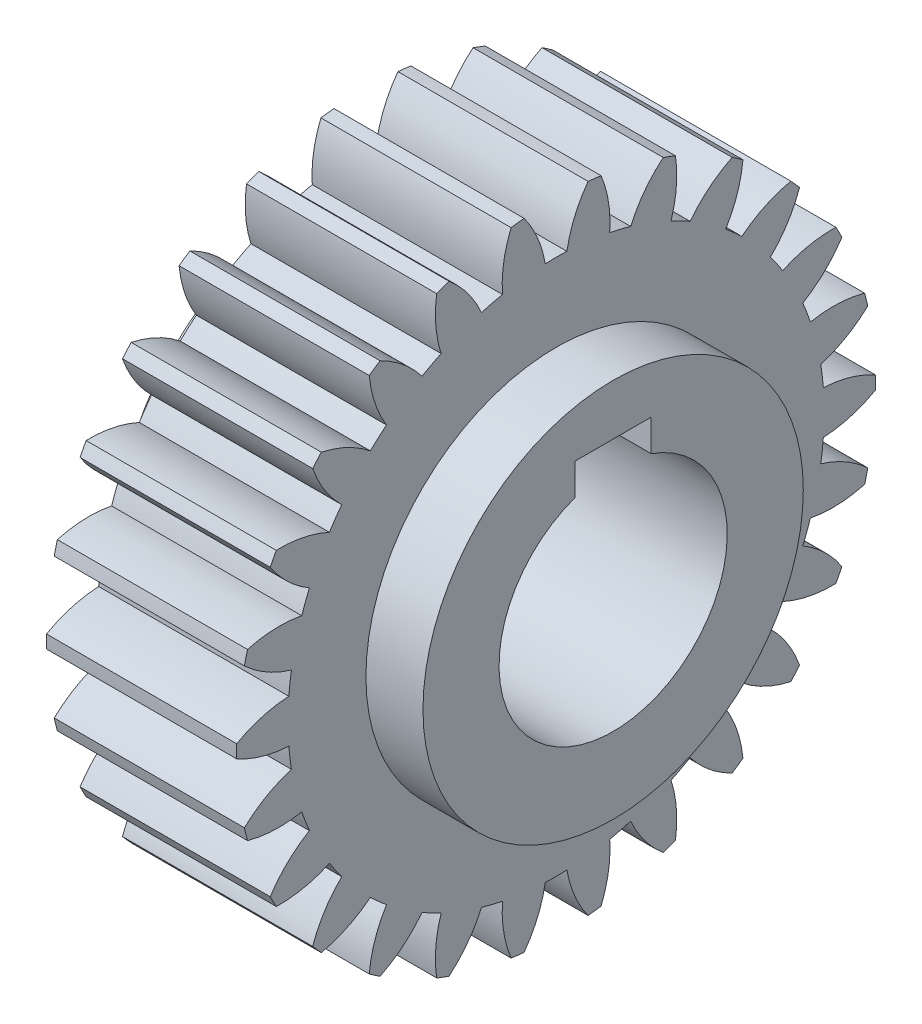
from build123d import *

# Parameters (mm, degrees)
BASPROSKE_W       = 25
BASPROSKE_H       = 42
TOOTHCUT_DEPTH    = 65.443773943
TEETHCUTS_COUNT   = 26
TEETHCUTS_ANGLE   = 346.153846154
HUBNEABOTSKE_R    = 25
HUBNEARBOTH_DEPTH = 7.5000254
HUBFAR_START      = 7.5000254
HUBFARSKE_R       = 25
HUBFAR_DEPTH      = 7.5000254
BORSKE_R          = 15
BORE_DEPTH        = 40.0000508
KEYSKE_W          = 10
KEYSKE_H          = 18.3
KEYWAY_DEPTH      = 40.0000508


with BuildPart() as part:
    # BasProSke → Base-Revolve (revolve)
    with BuildSketch(Plane(origin=(0, 0, 0), x_dir=(1, 0, 0), z_dir=(0, 1, 0)), mode=Mode.PRIVATE) as base_revolve_sk:
        with Locations((12.5, 21)):
            Rectangle(BASPROSKE_W, BASPROSKE_H)
    revolve(base_revolve_sk.sketch.rotate(Axis((-10, 0, 0), (1, 0, 0)), 180), axis=Axis((-10, 0, 0), (1, 0, 0)))

    # TooCutSke → ToothCut (cut, through all)
    with BuildSketch(Plane(origin=(0, 0, 0), x_dir=(0, 0, -1), z_dir=(1, 0, 0))):
        with BuildLine():
            ThreePointArc((1.420158149, 35.22037978), (0, 35.249), (-1.420158149, 35.22037978))
            ThreePointArc((-1.420158149, 35.22037978), (-2.438615981, 38.679606797), (-4.224127309, 41.812569804))
            ThreePointArc((-4.224127309, 41.812569804), (0, 42.0254), (4.224127309, 41.812569804))
            ThreePointArc((4.224127309, 41.812569804), (2.438615981, 38.679606797), (1.420158149, 35.22037978))
        make_face()
    toothcut = extrude(amount=TOOTHCUT_DEPTH, mode=Mode.SUBTRACT)

    # TeethCuts: ToothCut ×26 about axis
    teethcuts_axis = Axis((-10, 0, 0), (1, 0, 0))
    for i in range(1, TEETHCUTS_COUNT):
        add(toothcut.rotate(teethcuts_axis, i * TEETHCUTS_ANGLE / (TEETHCUTS_COUNT - 1)), mode=Mode.SUBTRACT)

    # HubNeaBotSke → HubNearBoth (add)
    with BuildSketch(Plane.ZY):
        with Locations(Location((0, 0, 0), (0, 0, 180))):
            Circle(HUBNEABOTSKE_R)
    extrude(amount=HUBNEARBOTH_DEPTH)

    # HubFarSke → HubFar (add)
    with BuildSketch(Plane(origin=(25, 0, 0), x_dir=(0, 0, -1), z_dir=(1, 0, 0)).offset(HUBFAR_START)):
        Circle(HUBFARSKE_R)
    extrude(amount=-HUBFAR_DEPTH)

    # BorSke → Bore (cut, symmetric)
    with BuildSketch(Plane(origin=(0, 0, 0), x_dir=(0, 0, -1), z_dir=(1, 0, 0))):
        with Locations(Location((0, 0, 0), (0, 0, 180))):
            Circle(BORSKE_R)
    extrude(amount=BORE_DEPTH, both=True, mode=Mode.SUBTRACT)

    # KeySke → Keyway (cut, symmetric)
    with BuildSketch(Plane(origin=(0, 0, 0), x_dir=(0, 0, -1), z_dir=(1, 0, 0))):
        with Locations((0, 9.15)):
            Rectangle(KEYSKE_W, KEYSKE_H)
    extrude(amount=KEYWAY_DEPTH, both=True, mode=Mode.SUBTRACT)


solid = part.part
